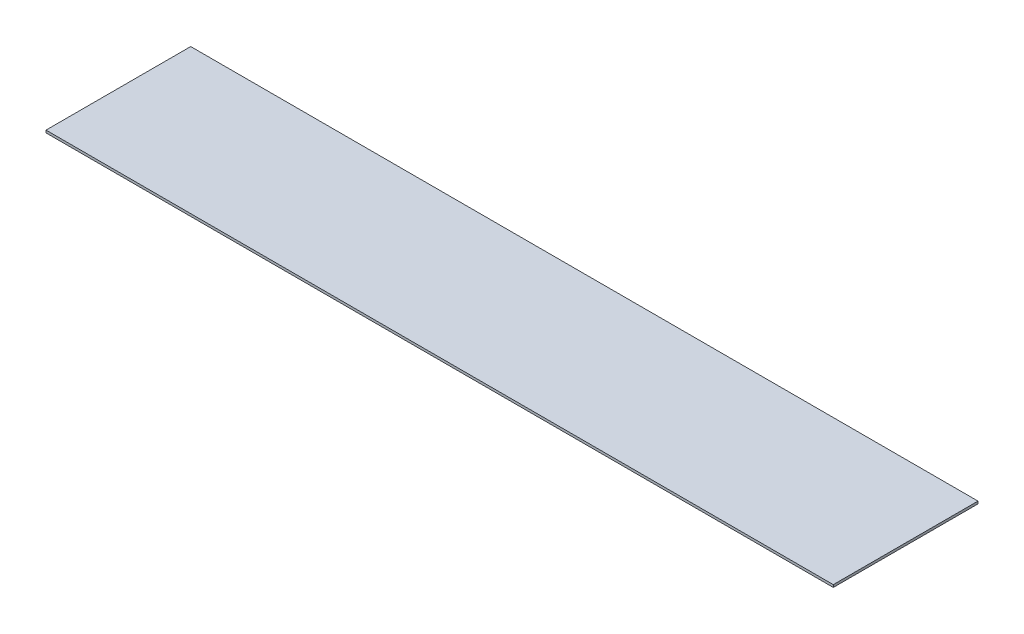
from build123d import *

# Parameters (mm, degrees)
SKETCH1_W           = 642
SKETCH1_H           = 118
BOSS_EXTRUDE1_DEPTH = 2


with BuildPart() as part:
    # Sketch1 → Boss-Extrude1 (new body)
    with BuildSketch(Plane(origin=(0, 0, 0), x_dir=(1, 0, 0), z_dir=(0, 1, 0))):
        Rectangle(SKETCH1_W, SKETCH1_H)
    extrude(amount=BOSS_EXTRUDE1_DEPTH)


solid = part.part
